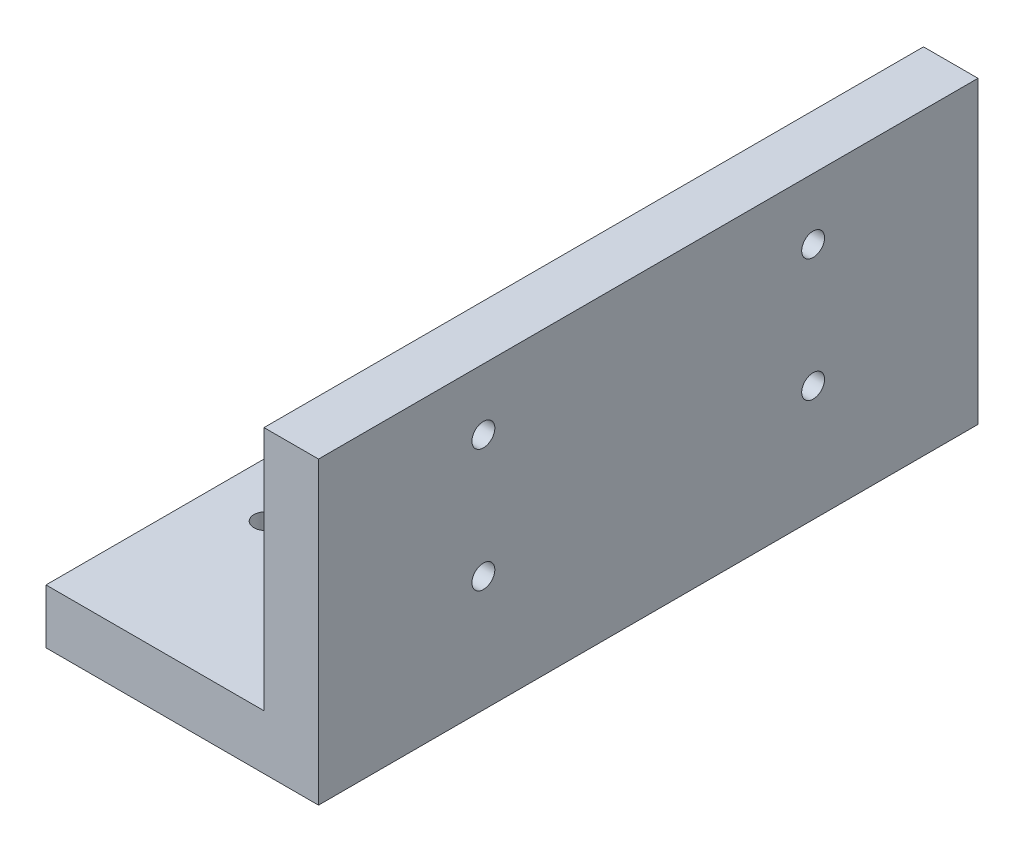
from build123d import *

# Parameters (mm, degrees)
EXTRUDE_1_DEPTH     = 121
CUT_EXTRUDE_2_REACH = 1320.001
SKETCH_3_R          = 2.099999998
SKETCH_3_R_2        = 2.100000002
SKETCH_5_R          = 2.1
CUT_EXTRUDE_3_DEPTH = 10


with BuildPart() as part:
    # 草图1 → 凸台-拉伸1 (new body)
    with BuildSketch(Plane.XY):
        Polygon((0, 24.51048951), (10, 24.51048951), (10, -30.48951049), (-40, -30.48951049), (-40, -20.48951049), (0, -20.48951049), align=None)
    extrude(amount=EXTRUDE_1_DEPTH)

    # 草图3 → 切除-拉伸2 (cut, up to next)
    with BuildSketch(Plane(origin=(-858.744003867, -20.48951049, -869.143932912), x_dir=(-1, 0, 0), z_dir=(0, 1, 0)), mode=Mode.PRIVATE) as cut_extrude_2_sk1:
        with Locations(Location((-848.744003867, 959.893932917, 0), (0, 0, 90))):
            Circle(SKETCH_3_R)
    cut_extrude_2_tool1 = extrude(cut_extrude_2_sk1.sketch, amount=-CUT_EXTRUDE_2_REACH, mode=Mode.PRIVATE) & part.part
    # 草图3 → 切除-拉伸2 (cut, up to next)
    with BuildSketch(Plane(origin=(-858.744003867, -20.48951049, -869.143932912), x_dir=(-1, 0, 0), z_dir=(0, 1, 0)), mode=Mode.PRIVATE) as cut_extrude_2_sk2:
        with Locations(Location((-828.744003867, 959.893932906, 0), (0, 0, 90))):
            Circle(SKETCH_3_R_2)
    cut_extrude_2_tool2 = extrude(cut_extrude_2_sk2.sketch, amount=-CUT_EXTRUDE_2_REACH, mode=Mode.PRIVATE) & part.part
    # 草图3 → 切除-拉伸2 (cut, up to next)
    with BuildSketch(Plane(origin=(-858.744003867, -20.48951049, -869.143932912), x_dir=(-1, 0, 0), z_dir=(0, 1, 0)), mode=Mode.PRIVATE) as cut_extrude_2_sk3:
        with Locations(Location((-828.744003867, 899.393932906, 0), (0, 0, 90))):
            Circle(SKETCH_3_R_2)
    cut_extrude_2_tool3 = extrude(cut_extrude_2_sk3.sketch, amount=-CUT_EXTRUDE_2_REACH, mode=Mode.PRIVATE) & part.part
    # 草图3 → 切除-拉伸2 (cut, up to next)
    with BuildSketch(Plane(origin=(-858.744003867, -20.48951049, -869.143932912), x_dir=(-1, 0, 0), z_dir=(0, 1, 0)), mode=Mode.PRIVATE) as cut_extrude_2_sk4:
        with Locations(Location((-848.744003867, 899.393932906, 0), (0, 0, 90))):
            Circle(SKETCH_3_R_2)
    cut_extrude_2_tool4 = extrude(cut_extrude_2_sk4.sketch, amount=-CUT_EXTRUDE_2_REACH, mode=Mode.PRIVATE) & part.part
    add(cut_extrude_2_tool1.solids().sort_by_distance((-10, -20.48951, 90.75))[0], mode=Mode.SUBTRACT)
    add(cut_extrude_2_tool2.solids().sort_by_distance((-30, -20.48951, 90.75))[0], mode=Mode.SUBTRACT)
    add(cut_extrude_2_tool3.solids().sort_by_distance((-30, -20.48951, 30.25))[0], mode=Mode.SUBTRACT)
    add(cut_extrude_2_tool4.solids().sort_by_distance((-10, -20.48951, 30.25))[0], mode=Mode.SUBTRACT)

    # 草图5 → 切除-拉伸3 (cut)
    with BuildSketch(Plane.ZY):
        with Locations((30.250000004, 13.26048951)):
            Circle(SKETCH_5_R)
        with Locations((30.250000004, -9.23951049)):
            Circle(SKETCH_5_R)
        with Locations((90.750000004, 13.26048951)):
            Circle(SKETCH_5_R)
        with Locations((90.750000004, -9.23951049)):
            Circle(SKETCH_5_R)
    extrude(amount=-CUT_EXTRUDE_3_DEPTH, mode=Mode.SUBTRACT)


solid = part.part
